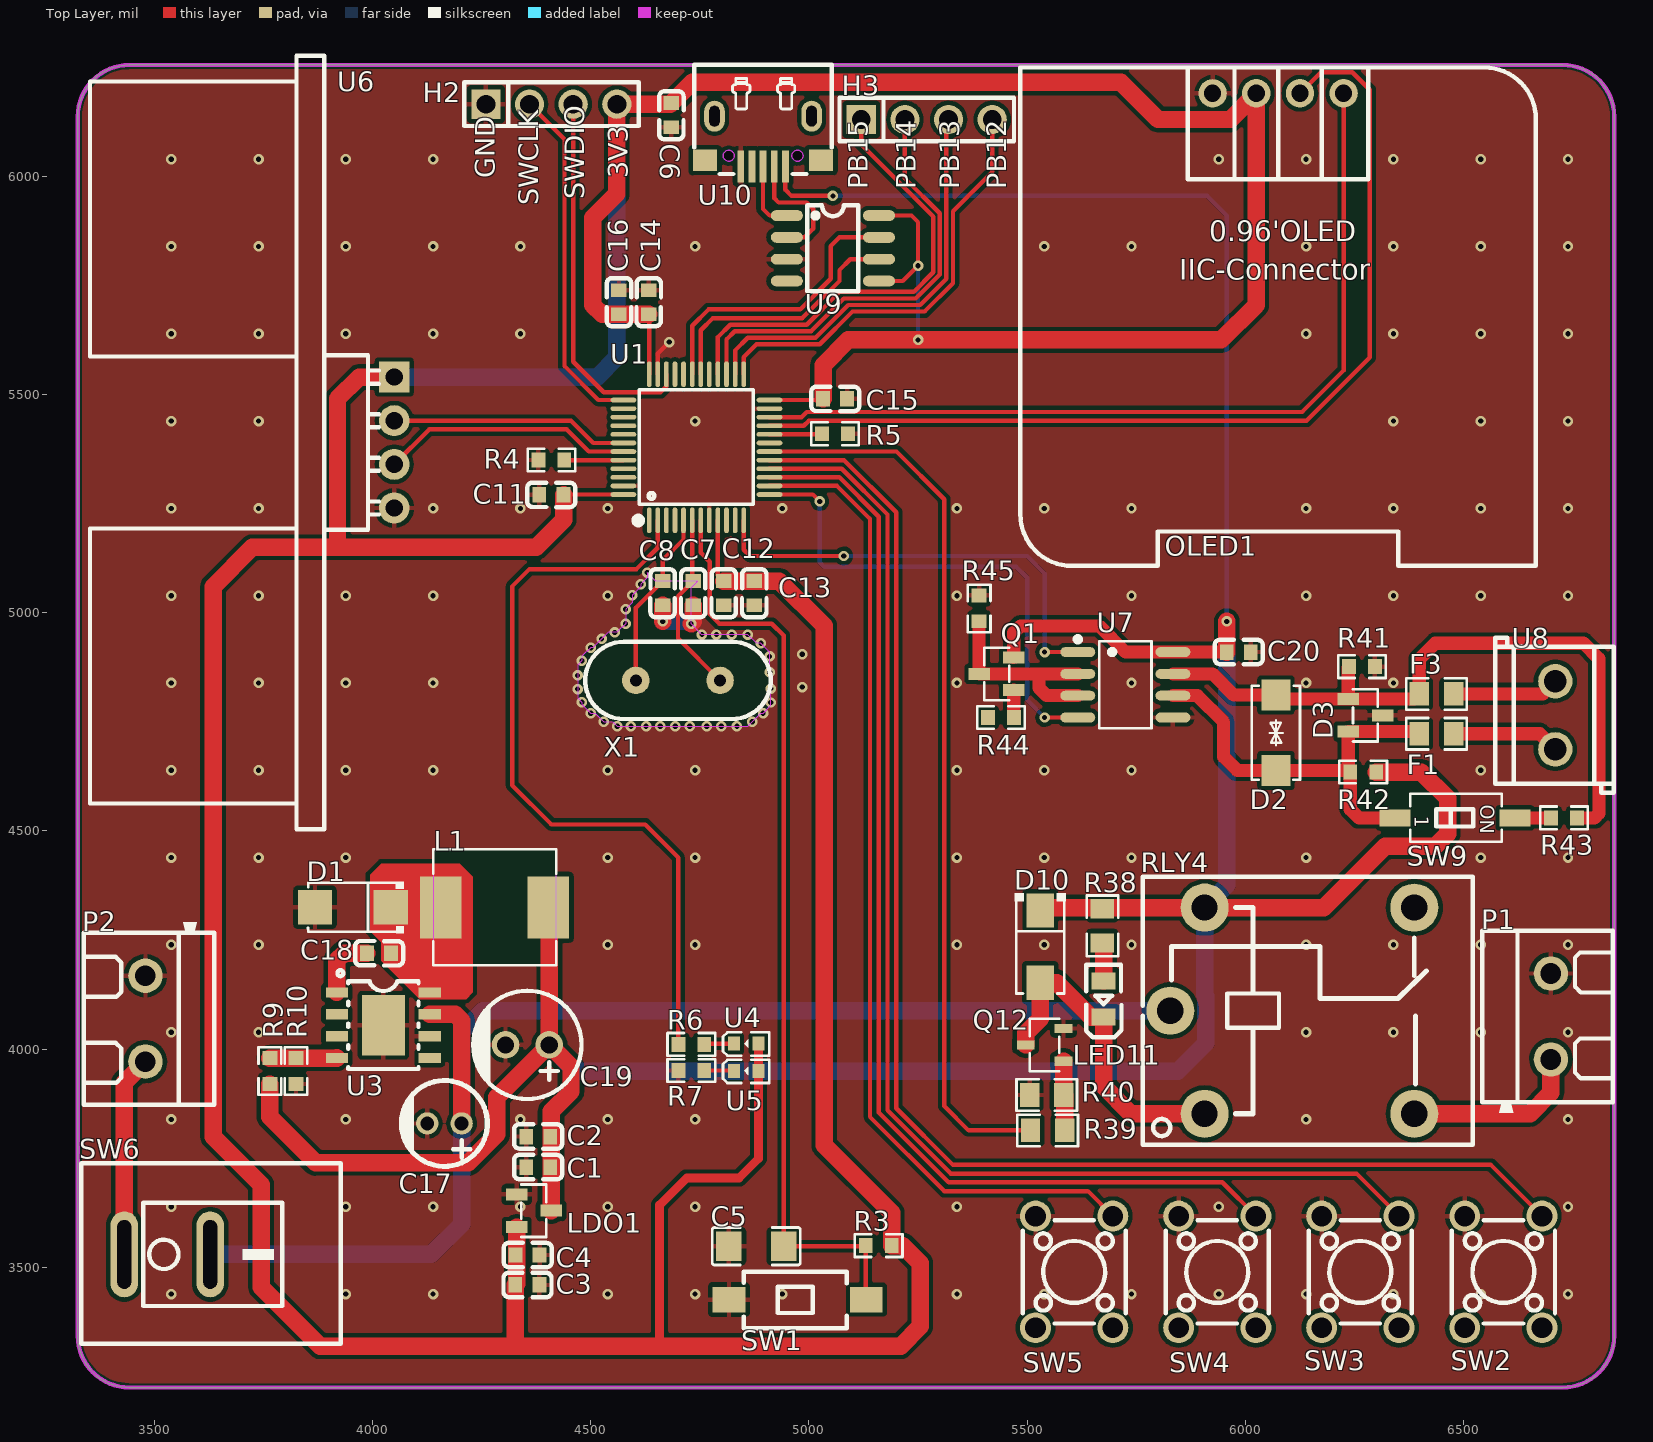
[diagram p0: Top Layer view]
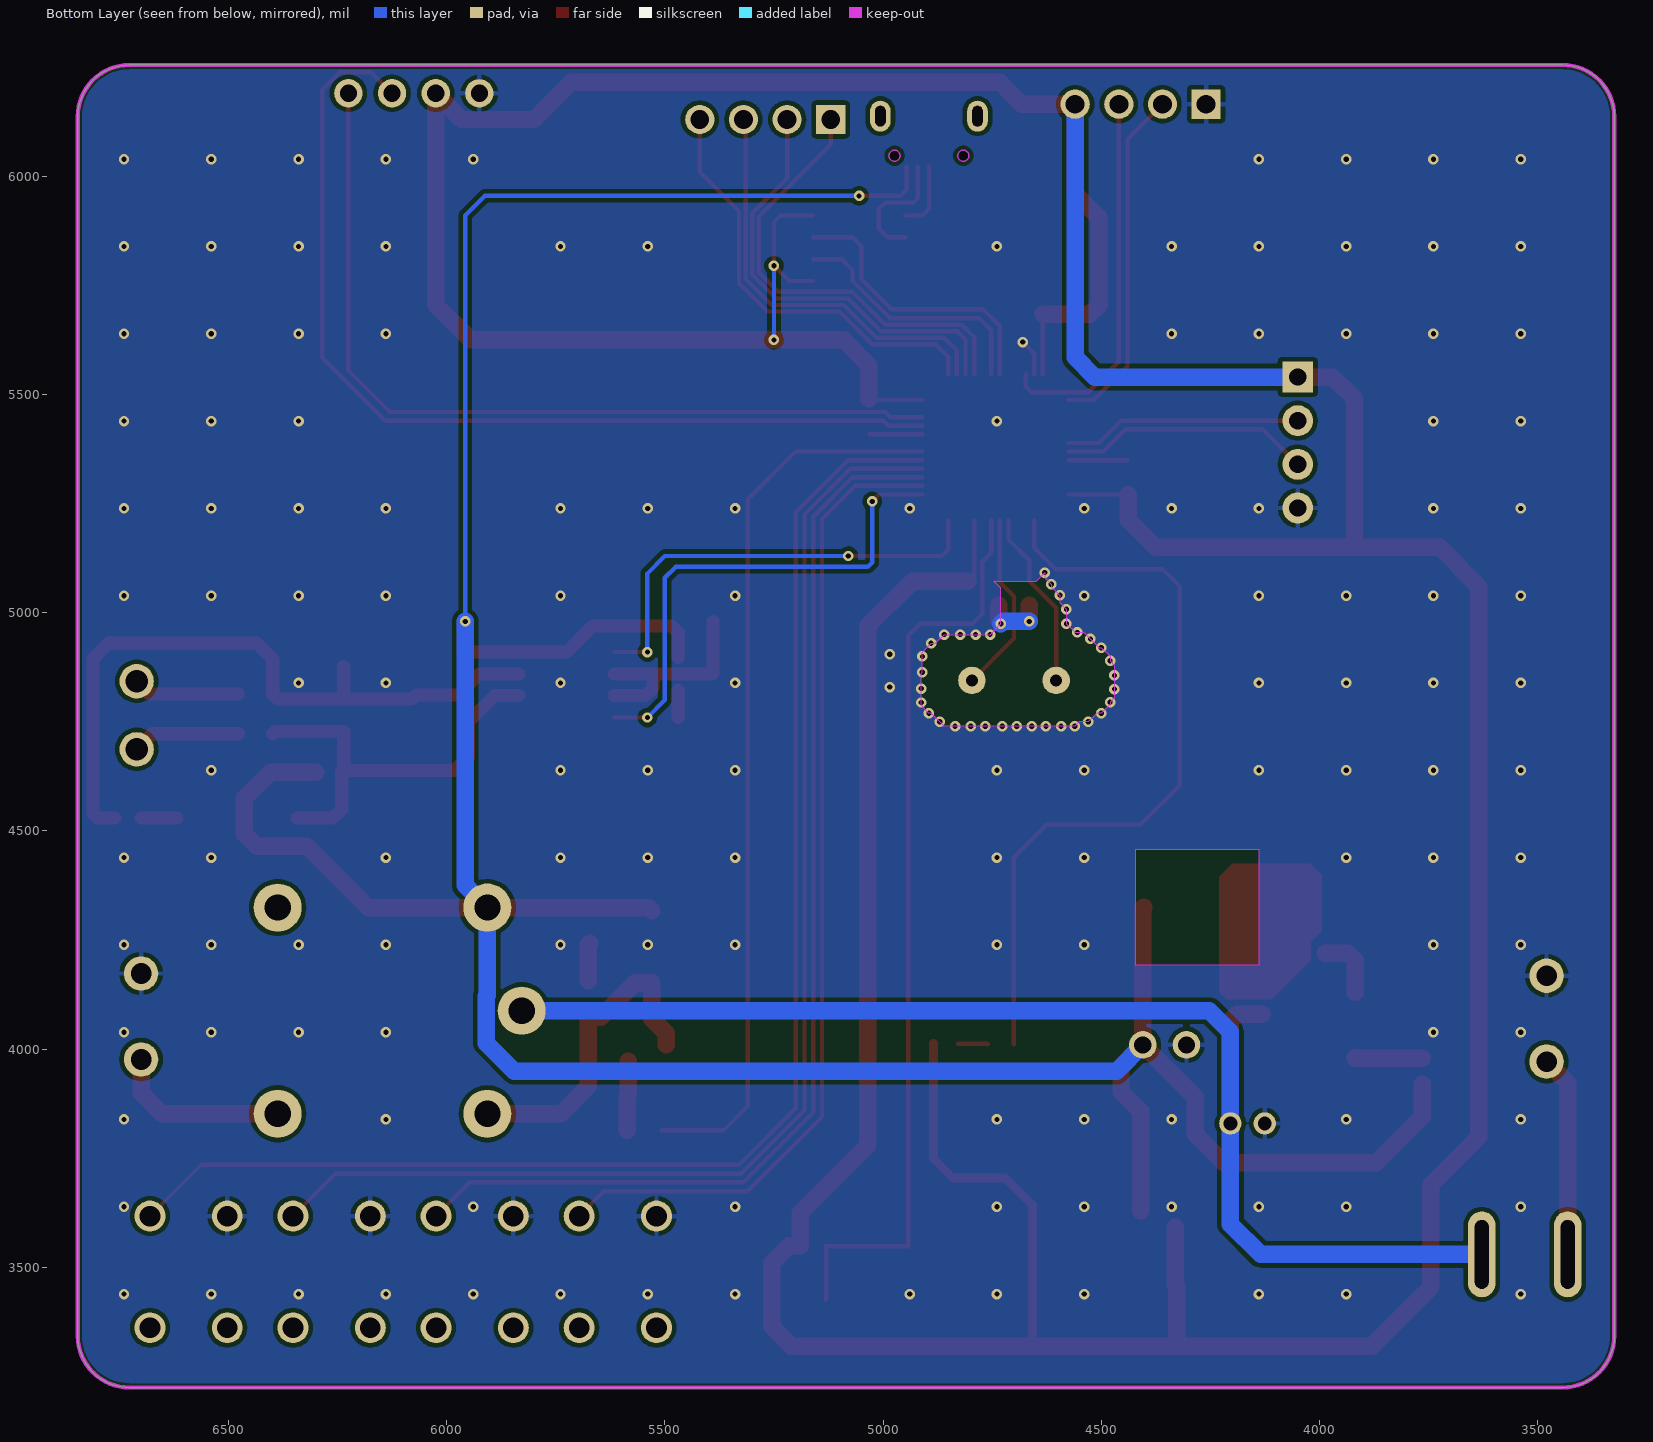
[diagram p1: Bottom Layer view, seen from below]
# Altium PCB MISC64779.pcbdoc
Units mil, origin at the board's own origin, x right, y up, seen from the top; angles counter-clockwise.
Board outline 3520 x 3030 mil, 2 copper layers (Top Layer, Bottom Layer), stack 62.206 mil thick; 67 components, 64 nets, 229 pads, 183 vias.

## Layer stack, top to bottom
Top Solder Mask Layer: solder mask 0.394, Dk 3.3
Top Layer: signal copper 1.379
Dielectric1: surface 59.449, FR4, Dk 4.5
Bottom Layer: signal copper 1.378
Bottom Solder Mask Layer: solder mask 0.394, Dk 3.3

## Board outline
3443.11,6255 ccw(c3443.11,6136.89) 3325,6136.89 3325,3343.11 ccw(c3443.11,3343.11) 3443.11,3225 6726.89,3225 ccw(c6726.89,3343.11) 6845,3343.11 6845,6136.89 ccw(c6726.89,6136.89) 6726.89,6255

## Design rules (kind name [scope] priority, off if disabled: settings)
BoardOutlineClearance copperThickness2oz_1 [All] p2 off: genericclearance=7.99 ignorepadtopadclearanceinfootprint=FALSE except(0: Arc-SplitContinuation Track-SplitContinuation SMDPad-SplitContinuation THPad-SplitContinuation Via-SplitContinuation Fill-SplitContinuation Region-SplitContinuation Poly-SplitContinuation Text-SplitContinuation Hole-SplitContinuation; 5.98: Arc-CutoutEdge Track-CutoutEdge SMDPad-CutoutEdge THPad-CutoutEdge Via-CutoutEdge Text-CutoutEdge; 6.9: Hole-OutlineEdge Hole-CutoutEdge; 10: Poly-OutlineEdge Poly-CutoutEdge; 11.81: Arc-OutlineEdge Track-OutlineEdge SMDPad-OutlineEdge THPad-OutlineEdge Via-OutlineEdge Fill-OutlineEdge Region-OutlineEdge Text-OutlineEdge Fill-CutoutEdge Region-CutoutEdge)
BoardOutlineClearance Plane_innerPlane_1 [All] p4 off: genericclearance=4.02 ignorepadtopadclearanceinfootprint=FALSE except(0: Arc-SplitContinuation Track-SplitContinuation SMDPad-SplitContinuation THPad-SplitContinuation Via-SplitContinuation Fill-SplitContinuation Region-SplitContinuation Poly-SplitContinuation Text-SplitContinuation Hole-SplitContinuation; 5.98: Arc-CutoutEdge Track-CutoutEdge SMDPad-CutoutEdge THPad-CutoutEdge Via-CutoutEdge Text-CutoutEdge; 6.9: Hole-OutlineEdge Hole-CutoutEdge; 10: Poly-OutlineEdge Poly-CutoutEdge; 11.81: Arc-OutlineEdge Track-OutlineEdge SMDPad-OutlineEdge THPad-OutlineEdge Via-OutlineEdge Fill-OutlineEdge Region-OutlineEdge Text-OutlineEdge Fill-CutoutEdge Region-CutoutEdge)
BoardOutlineClearance Copper_copperRegion_1 [All] p6 off: genericclearance=4.02 ignorepadtopadclearanceinfootprint=FALSE except(0: Arc-SplitContinuation Track-SplitContinuation SMDPad-SplitContinuation THPad-SplitContinuation Via-SplitContinuation Fill-SplitContinuation Region-SplitContinuation Poly-SplitContinuation Text-SplitContinuation Hole-SplitContinuation; 5.98: Arc-CutoutEdge Track-CutoutEdge SMDPad-CutoutEdge THPad-CutoutEdge Via-CutoutEdge Text-CutoutEdge; 6.9: Hole-OutlineEdge Hole-CutoutEdge; 10: Poly-OutlineEdge Poly-CutoutEdge; 11.81: Arc-OutlineEdge Track-OutlineEdge SMDPad-OutlineEdge THPad-OutlineEdge Via-OutlineEdge Fill-OutlineEdge Region-OutlineEdge Text-OutlineEdge Fill-CutoutEdge Region-CutoutEdge)
BoardOutlineClearance copperThickness1oz_1 [All] p8: genericclearance=4.02 ignorepadtopadclearanceinfootprint=FALSE except(0: Arc-SplitContinuation Track-SplitContinuation SMDPad-SplitContinuation THPad-SplitContinuation Via-SplitContinuation Fill-SplitContinuation Region-SplitContinuation Poly-SplitContinuation Text-SplitContinuation Hole-SplitContinuation; 5.98: Arc-CutoutEdge Track-CutoutEdge SMDPad-CutoutEdge THPad-CutoutEdge Via-CutoutEdge Text-CutoutEdge; 6.9: Hole-OutlineEdge Hole-CutoutEdge; 10: Poly-OutlineEdge Poly-CutoutEdge; 11.81: Arc-OutlineEdge Track-OutlineEdge SMDPad-OutlineEdge THPad-OutlineEdge Via-OutlineEdge Fill-OutlineEdge Region-OutlineEdge Text-OutlineEdge Fill-CutoutEdge Region-CutoutEdge)
Clearance copperThickness2oz [All] p1 off: gap=7.99 ignorepadtopadclearanceinfootprint=FALSE except(5.98: SMDPad-Track SMDPad-SMDPad THPad-Track SMDPad-THPad THPad-THPad Track-Via SMDPad-Via THPad-Via Via-Via Fill-SMDPad Region-SMDPad Fill-THPad Region-THPad Fill-Via Region-Via Fill-Fill Fill-Region Region-Region Arc-Track Arc-SMDPad Arc-THPad Arc-Via Fill-Arc Region-Arc Arc-Arc Text-Track SMDPad-Text Text-THPad Text-Via Fill-Text Region-Text Arc-Text Text-Text; 6.9: Hole-Track Hole-SMDPad Hole-THPad Hole-Via Fill-Hole Region-Hole Hole-Arc Hole-Text; 10: Poly-Track Poly-SMDPad Poly-THPad Poly-Via Poly-Fill Poly-Region Poly-Poly Poly-Arc Poly-Text Poly-Hole; 11.81: Fill-Track Region-Track)
Clearance Plane_innerPlane [All] p3 off: gap=4.02 ignorepadtopadclearanceinfootprint=FALSE except(5.98: SMDPad-Track SMDPad-SMDPad THPad-Track SMDPad-THPad THPad-THPad Track-Via SMDPad-Via THPad-Via Via-Via Fill-SMDPad Region-SMDPad Fill-THPad Region-THPad Fill-Via Region-Via Fill-Fill Fill-Region Region-Region Arc-Track Arc-SMDPad Arc-THPad Arc-Via Fill-Arc Region-Arc Arc-Arc Text-Track SMDPad-Text Text-THPad Text-Via Fill-Text Region-Text Arc-Text Text-Text; 6.9: Hole-Track Hole-SMDPad Hole-THPad Hole-Via Fill-Hole Region-Hole Hole-Arc Hole-Text; 10: Poly-Track Poly-SMDPad Poly-THPad Poly-Via Poly-Fill Poly-Region Poly-Poly Poly-Arc Poly-Text Poly-Hole; 11.81: Fill-Track Region-Track)
Clearance Copper_copperRegion [All] p5 off: gap=4.02 ignorepadtopadclearanceinfootprint=FALSE except(5.98: SMDPad-Track SMDPad-SMDPad THPad-Track SMDPad-THPad THPad-THPad Track-Via SMDPad-Via THPad-Via Via-Via Fill-SMDPad Region-SMDPad Fill-THPad Region-THPad Fill-Via Region-Via Fill-Fill Fill-Region Region-Region Arc-Track Arc-SMDPad Arc-THPad Arc-Via Fill-Arc Region-Arc Arc-Arc Text-Track SMDPad-Text Text-THPad Text-Via Fill-Text Region-Text Arc-Text Text-Text; 6.9: Hole-Track Hole-SMDPad Hole-THPad Hole-Via Fill-Hole Region-Hole Hole-Arc Hole-Text; 10: Poly-Track Poly-SMDPad Poly-THPad Poly-Via Poly-Fill Poly-Region Poly-Poly Poly-Arc Poly-Text Poly-Hole; 11.81: Fill-Track Region-Track)
Clearance copperThickness1oz [All] p7: gap=4.02 ignorepadtopadclearanceinfootprint=FALSE except(5.98: SMDPad-Track SMDPad-SMDPad THPad-Track SMDPad-THPad THPad-THPad Track-Via SMDPad-Via THPad-Via Via-Via Fill-SMDPad Region-SMDPad Fill-THPad Region-THPad Fill-Via Region-Via Fill-Fill Fill-Region Region-Region Arc-Track Arc-SMDPad Arc-THPad Arc-Via Fill-Arc Region-Arc Arc-Arc Text-Track SMDPad-Text Text-THPad Text-Via Fill-Text Region-Text Arc-Text Text-Text; 6.9: Hole-Track Hole-SMDPad Hole-THPad Hole-Via Fill-Hole Region-Hole Hole-Arc Hole-Text; 10: Poly-Track Poly-SMDPad Poly-THPad Poly-Via Poly-Fill Poly-Region Poly-Poly Poly-Arc Poly-Text Poly-Hole; 11.81: Fill-Track Region-Track)
DiffPairsRouting differentialPair [All] p1: maxlimit=6 minlimit=6 mostfreqgap=6 toplayer_minwidth=5 toplayer_prefwidth=10 toplayer_maxwidth=100 toplayer_mingap=6 toplayer_prefgap=6 toplayer_maxgap=6 bottomlayer_minwidth=5 bottomlayer_prefwidth=10 bottomlayer_maxwidth=100 bottomlayer_mingap=6 bottomlayer_prefgap=6 bottomlayer_maxgap=6 maxuncoupledlength=10
HoleToHoleClearance otherClearance [All] p1: gap=11.81 allowstackedmicrovias=TRUE
Length netLength [All] p1: minlimit=0 maxlimit=0
PasteMaskExpansion pasteMaskExpansion [All] p1: expansion=0
PlaneConnect innerPlane [All] p1: planeconnectstyle=Relief reliefexpansion=20 reliefentries=4 reliefconductorwidth=10 reliefairgap=10
PolygonConnect copperRegion [All] p1: connectstyle=Relief reliefconductorwidth=10 reliefentries=4 polygonreliefangle="90 Angle" airgapwidth=10 via.connectstyle=Relief via.reliefconductorwidth=10 via.reliefentries=4 via.polygonreliefangle="90 Angle" via.airgapwidth=10
RoutingVias viaSize [All] p1: holewidth=12.01 width=24.02 viastyle="Through Hole" minholewidth=11.81 minwidth=19.68 maxholewidth=248.03 maxwidth=393.7
SolderMaskExpansion solderMaskExpansion [IsVia] p1: expansion=-1000 istentingtop=TRUE
SolderMaskExpansion solderMaskExpansion [All] p2: expansion=2 istentingtop=FALSE
Width copperThickness2oz_2 [All] p1 off: maxlimit=100 minlimit=8 preferedwidth=10
Width copperThickness1oz_2 [All] p2: maxlimit=100 minlimit=5 preferedwidth=10

## Components (designator, comment, footprint, x,y, rotation, side; value= is the part's Value field where it differs from the comment)
C1 "10uF" C0603 4380,3730 r0 top
C2 "100nF" C0603 4380,3800 r0 top
C3 "100nF" C0603 4355,3460 r180 top
C4 "10uF" C0603 4355.51,3528.58 r180 top
C5 "100uF" C1206 4879.43,3548.58 r0 top
C6 "100nF" C0603 4685,6140 r90 top
C7 "20pF" C0603 4735,5045 r90 top
C8 "20pF" C0603 4665,5045 r90 top
C11 "100nF" C0603 4410,5270 r0 top
C12 "100nF" C0603 4805,5045 r90 top
C13 "100nF" C0603 4875,5045 r90 top
C14 "100nF" C0603 4632.98,5711.29 r270 top
C15 "100nF" C0603 5060,5490 r180 top
C16 "4.7nF" C0603 4564.8,5711.29 r270 top
C17 "10uF" CAP-TH_BD5.0-P2.00-D0.8-FD 4165,3830 r180 top
C18 "10nF" C0603 4015,4220 r180 top
C19 "220uF" CAP-TH_BD6.3-P2.50-D1.0-FD 4355,4010 r180 top
C20 "100nF" C0603 5985,4910 r0 top
D1 "B340A" SMA_L4.3-W2.6-LS5.1-RD 3955,4325 r180 top
D2 "SMAJ7.0CA" SMA_L4.5-W2.7-LS5.1-BI 6070,4725 r270 top
D3 "SM712" SOT-23-3_L2.9-W1.3-P1.90-LS2.4-BR 6275,4765 r180 top
D10 "1N4007" SMA_L4.3-W2.5-LS5.0-RD 5530,4235 r270 top
F1 "0R" R0805 6437.63,4722.67 r0 top
F3 "0R" R0805 6437.63,4814.14 r0 top
H2 "" HDR-TH_4P-P2.54-V-M 4410,6165 r0 top
H3 "" HDR-TH_4P-P2.54-V-M 5270,6130 r0 top
L1 "15uH" IND-SMD_L7.0-W6.6_FXL0630 4280,4325 r0 top
LDO1 "SC662K-3.3V" SOT-23-3_L2.9-W1.3-P1.90-LS2.4-BR 4370,3630 r180 top
LED11 "NCD0805R1" LED0805-R-RD 5675,4115 r90 top
OLED1 "" 0.96OLED_4P 6075,6190 r0 top
P1 "KF301-2P terminal block" CONN-TH_XY301V-A-5.0-2P 6700,4075 r270 top
P2 "KF301-2P terminal block" CONN-TH_XY301V-A-5.0-2P 3480,4070 r90 top
Q1 "S8550-2TY" SOT-23-3_L2.9-W1.3-P0.95-LS2.4-BR 5430,4860 r0 top
Q12 "S8050 J3Y(RANGE:200-350)" SOT-23-3_L3.0-W1.7-P0.95-LS2.9-BR 5540,4010 r0 top
R3 "1kΩ" R0603 5160,3550 r0 top
R4 "10kΩ" R0603 4410,5350 r0 top
R5 "10kΩ" R0603 5060,5410 r180 top
R6 "510Ω" R0603 4730.72,4011.18 r180 top
R7 "510Ω" R0603 4730.72,3951.18 r180 top
R9 "10kΩ" R0603 3765,3950 r90 top
R10 "3.24kΩ" R0603 3825,3950 r90 top
R38 "1.5kΩ" R0805 5672.28,4282.73 r90 top
R39 "1kΩ" R0805 5547.1,3814.1 r0 top
R40 "10kΩ" R0805 5545,3895 r0 top
R41 "3.3K" R0603 6266.95,4876.44 r180 top
R42 "3.3K" R0603 6270,4635 r0 top
R43 "120R" R0603 6730,4530 r0 top
R44 "4.7K" R0603 5440,4760 r0 top
R45 "10K" R0603 5390,5010 r90 top
RLY4 "SRD-05VDC-SL-C" RELAY-TH_SRD-XXVDC-XL-C 6107.46,4088.36 r0 top
SW1 "TS-1101-C-W" SW-SMD_L6.0-W3.3-LS8.0 4974.3,3426.3 r0 top
SW2 "" SW-TH_4P-L6.0-W6.0-P4.50-LS6.5 6591.06,3489.8 r270 top
SW3 "" SW-TH_4P-L6.0-W6.0-P4.50-LS6.5 6263.31,3489.8 r270 top
SW4 "" SW-TH_4P-L6.0-W6.0-P4.50-LS6.5 5935.55,3489.8 r270 top
SW5 "" SW-TH_4P-L6.0-W6.0-P4.50-LS6.5 5607.79,3489.8 r270 top
SW6 "KCD11-2P-R" SW-TH_2P-L15.0-W10.5-P5.00_KCD11-2P-R 3530,3530 r0 top
SW9 "ZX-1.27BM-1PSMD" SW-SMD_L5.4-W2.8-LS8.2 6480,4530 r270 top
U1 "STM32F103C8T6" LQFP-48_L7.0-W7.0-P0.50-LS9.0-BL 4742.36,5379.1 r0 top
U3 "TPS5430DDAR" ESOP-8_L4.9-W3.9-P1.27-LS6.0-TL-EP 4025,4055 r0 top
U4 "42-51/GHC-YW2X2K/3T" LED-SMD_L1.6-W0.8-FD_GREEN-1 4856.42,4012.9 r180 top
U5 "42-51/GHC-YW2X2K/3T" LED-SMD_L1.6-W0.8-FD_GREEN-1 4856.42,3950.25 r180 top
U6 "HC-SR04" TH_HC-SR04V 4050,5390 r270 top
U7 "MAX485ESA" SOP-8_L5.0-W4.0-P1.27-LS6.0-BL 5725,4835 r270 top
U8 "KF396-3.96-2P" CONN-TH_P3.96_KF396-3.96-2P 6710,4765 r90 top
U9 "CH340N" SOP-8_L4.9-W3.9-P1.27-LS6.0-BL 5055,5835 r270 top
U10 "micro-B USB socket" MICRO-USB_C9900039549 4895,6080 r180 top
X1 "8MHz" OSC-TH_L10.0-W4.5-P5.00 4700,4845 r90 top

## Footprints (in the part's own frame and the unit in brackets; to place one, negate y for a bottom-side part, rotate by r counter-clockwise, add the part's x,y. Pads: shape width x height; smd on the part's side, far side on the other; paste and mask are expansions set on the pad)
0.96OLED_4P [mm]
  round 1.65 hole 1 copper offset 0,0: 1(-3.81,-0.001) 2(-1.27,0.002) 3(1.27,0.002) 4(3.81,0.002)
  silkscreen extent -15,-27.5 15,1.5
C0603 [mm]
  rect 0.8x0.9 smd: 1(-0.7,0) 2(0.7,0)
  silkscreen extent -1.41,-0.71 1.39,0.72
C1206 [mm]
  rect 1.485x1.728 smd paste-100 mask+0.051: 1(-1.593,0) 2(1.593,0)
  silkscreen extent -2.56,-1.09 2.56,1.09
CAP-TH_BD5.0-P2.00-D0.8-FD [mm]
  round 1.3 hole 0.8: 1(-1,0) 2(1,0)
  silkscreen extent -2.5,-2.5 2.5,2.5
CAP-TH_BD6.3-P2.50-D1.0-FD [mm]
  round 1.6 hole 1: 1(-1.27,0) 2(1.27,0)
  silkscreen extent -3.15,-3.15 3.17,3.15
CONN-TH_P3.96_KF396-3.96-2P [mm]
  round 2 hole 1.3: 1(-1.98,0) 2(1.98,0)
  silkscreen extent -4.51,-3.4 4.51,3.5
CONN-TH_XY301V-A-5.0-2P [mm]
  round 2 hole 1.2: 1(-2.5,0) 2(2.5,0)
  silkscreen extent -5,-4 5.6,3.6
ESOP-8_L4.9-W3.9-P1.27-LS6.0-TL-EP [mm]
  rect 1.3x0.6 smd: 1(-2.7,1.905) 2(-2.7,0.635) 3(-2.7,-0.635) 4(-2.7,-1.905) 5(2.7,-1.905) 6(2.7,-0.635) 7(2.7,0.635) 8(2.7,1.905)
  rect 2.5x3.5 smd: 9(0,0)
  silkscreen extent -2.67,-2.55 2.05,3.2
HDR-TH_4P-P2.54-V-M [mm]
  rect 1.7x1.7 hole 1.1: 1(-3.81,0)
  round 1.7 hole 1.1: 2(-1.27,0) 3(1.27,0) 4(3.81,0)
  silkscreen extent -5.08,-1.27 5.08,1.27
IND-SMD_L7.0-W6.6_FXL0630 [mm]
  rect 2.424x3.62 smd: 1(3.128,0) 2(-3.128,0)
  silkscreen extent -3.58,-3.38 3.58,3.38
LED0805-R-RD [mm]
  rect 1x1.4 smd: 1(1.05,0) 2(-1.05,0)
  silkscreen extent -2.22,-1.04 1.99,1.01
LED-SMD_L1.6-W0.8-FD_GREEN-1 [mm]
  rect 0.7x0.8 smd: 1(-0.715,0) 2(0.715,0)
  silkscreen extent -1.35,-0.65 1.35,0.7
LQFP-48_L7.0-W7.0-P0.50-LS9.0-BL [mm]
  oval 0.27x1.5 smd paste+0 mask+0.05: 1(-2.75,-4.25) 2(-2.25,-4.25) 3(-1.75,-4.25) 4(-1.25,-4.25) 5(-0.75,-4.25) 6(-0.25,-4.25) 7(0.25,-4.25) 8(0.75,-4.25) 9(1.25,-4.25) 10(1.75,-4.25) 11(2.25,-4.25) 12(2.75,-4.25) 25(2.75,4.25) 26(2.25,4.25) 27(1.75,4.25) 28(1.25,4.25) 29(0.75,4.25) 30(0.25,4.25) 31(-0.25,4.25) 32(-0.75,4.25) 33(-1.25,4.25) 34(-1.75,4.25) 35(-2.25,4.25) 36(-2.75,4.25)
  oval 1.5x0.27 smd paste+0 mask+0.05: 13(4.25,-2.75) 14(4.25,-2.25) 15(4.25,-1.75) 16(4.25,-1.25) 17(4.25,-0.75) 18(4.25,-0.25) 19(4.25,0.25) 20(4.25,0.75) 21(4.25,1.25) 22(4.25,1.75) 23(4.25,2.25) 24(4.25,2.75) 37(-4.25,2.75) 38(-4.25,2.25) 39(-4.25,1.75) 40(-4.25,1.25) 41(-4.25,0.75) 42(-4.25,0.25) 43(-4.25,-0.25) 44(-4.25,-0.75) 45(-4.25,-1.25) 46(-4.25,-1.75) 47(-4.25,-2.25) 48(-4.25,-2.75)
  silkscreen extent -3.59,-4.46 3.3,3.34
MICRO-USB_C9900039549 [mm]
  rect 0.4x1.85 smd paste-100 mask+0.051: 1(-1.3,1.462) 2(-0.65,1.462) 3(0,1.462) 4(0.65,1.462) 5(1.3,1.462)
  rect 1.4x1.25 smd paste-100 mask+0.051: 6(-3.375,1.1) 7(3.375,1.1)
  oval 1.2x1.8 hole 0.6 slot 1.2 at 90 deg copper offset -0.001,0.001: 6(-2.824,-1.463)
  oval 1.2x1.8 hole 0.6 slot 1.2 at 90 deg copper offset -0.001,-0.001: 7(2.826,-1.462)
  Board Outline Layer circle w0.003: c2,0.837 r0.325
  Board Outline Layer circle w0.003: c-2,0.837 r0.325
  Board Outline Layer region: 1.675,0.837 1.707,0.978 1.797,1.091 1.928,1.154 2.072,1.154 2.203,1.091 2.293,0.978 2.325,0.837 2.325,0.837 2.293,0.696 2.203,0.583 2.072,0.52 1.928,0.52 1.797,0.583 1.707,0.696 1.675,0.837
  Board Outline Layer region: 1.675,0.837 1.684,0.915 1.712,0.988 1.757,1.053 1.815,1.105 1.885,1.141 1.961,1.16 2.039,1.16 2.115,1.141 2.185,1.105 2.243,1.053 2.288,0.988 2.316,0.915 2.325,0.837 2.316,0.76 2.288,0.686 2.243,0.622 2.185,0.57 2.115,0.533 2.039,0.515 1.961,0.515 1.885,0.533 1.815,0.57 1.757,0.622 1.712,0.686 1.684,0.76
  Board Outline Layer region: -2.325,0.837 -2.293,0.978 -2.203,1.091 -2.072,1.154 -1.928,1.154 -1.797,1.091 -1.707,0.978 -1.675,0.837 -1.675,0.837 -1.707,0.696 -1.797,0.583 -1.928,0.52 -2.072,0.52 -2.203,0.583 -2.293,0.696 -2.325,0.837
  Board Outline Layer region: -2.325,0.837 -2.316,0.915 -2.288,0.988 -2.243,1.053 -2.185,1.105 -2.115,1.141 -2.039,1.16 -1.961,1.16 -1.885,1.141 -1.815,1.105 -1.757,1.053 -1.712,0.988 -1.684,0.915 -1.675,0.837 -1.684,0.76 -1.712,0.686 -1.757,0.622 -1.815,0.57 -1.885,0.533 -1.961,0.515 -2.039,0.515 -2.115,0.533 -2.185,0.57 -2.243,0.622 -2.288,0.686 -2.316,0.76
  Multi-Layer board cut-out: 1.675,0.837 1.707,0.978 1.797,1.091 1.928,1.154 2.072,1.154 2.203,1.091 2.293,0.978 2.325,0.837 2.325,0.837 2.293,0.696 2.203,0.583 2.072,0.52 1.928,0.52 1.797,0.583 1.707,0.696 1.675,0.837
  Multi-Layer board cut-out: -2.325,0.837 -2.293,0.978 -2.203,1.091 -2.072,1.154 -1.928,1.154 -1.797,1.091 -1.707,0.978 -1.675,0.837 -1.675,0.837 -1.707,0.696 -1.797,0.583 -1.928,0.52 -2.072,0.52 -2.203,0.583 -2.293,0.696 -2.325,0.837
  silkscreen extent -4,-4.46 4,1.91
OSC-TH_L10.0-W4.5-P5.00 [mm]
  round 1.6 hole 0.7: 1(0,2.45) 2(0,-2.45)
  silkscreen extent -2.25,-5.39 2.25,5.39
R0603 [mil]
  rect 31.75x34.02 smd paste-3937.01 mask+2: 1(-29.66,0) 2(29.66,0)
  silkscreen extent -55,-26 55,26
R0805 [mm]
  rect 1.133x1.377 smd paste-100 mask+0.051: 1(-1,0) 2(1,0)
  silkscreen extent -1.76,-0.92 1.76,0.92
RELAY-TH_SRD-XXVDC-XL-C [mil]
  round 110 hole 60: 1(-200.79,-236.22) 2(279.53,-236.2) 3(279.53,236.2) 4(-200.79,236.22) 5(-279.53,0)
  silkscreen extent -342,-307 413,307
SMA_L4.3-W2.5-LS5.0-RD [mm]
  rect 2x1.593 smd: 1(-2.1,0) 2(2.1,0)
  silkscreen extent -3.11,-1.48 2.73,1.48
SMA_L4.3-W2.6-LS5.1-RD [mm]
  rect 2x2 smd: 1(-2.2,0) 2(2.2,0)
  silkscreen extent -2.98,-1.5 2.6,1.5
SMA_L4.5-W2.7-LS5.1-BI [mm]
  rect 1.8x1.7 smd: 1(-2.192,0) 2(2.192,0)
  silkscreen extent -2.73,-1.4 2.73,1.4
SOP-8_L4.9-W3.9-P1.27-LS6.0-BL [mm]
  oval 0.63x1.865 smd: 1(-1.905,-2.682) 2(-0.635,-2.682) 3(0.635,-2.682) 4(1.905,-2.682) 5(1.905,2.682) 6(0.635,2.682) 7(-0.635,2.682) 8(-1.905,2.682)
  silkscreen extent -2.5,-1.5 2.5,1.48
SOP-8_L5.0-W4.0-P1.27-LS6.0-BL [mil]
  oval 22.6x80.14 smd: 1(-75,-108.97) 2(-25,-108.97) 3(25,-108.97) 4(75,-108.97) 5(75,108.97) 6(25,108.97) 7(-25,108.97) 8(-75,108.97)
  silkscreen extent -110,-115 99,60
SOT-23-3_L2.9-W1.3-P0.95-LS2.4-BR [mm]
  rect 1.25x0.7 smd: 1(1,-0.95) 2(1,0.95) 3(-1,0)
  silkscreen extent -0.73,-1.53 0.73,1.53
SOT-23-3_L2.9-W1.3-P1.90-LS2.4-BR [mm]
  rect 1.25x0.7 smd: 1(1,-0.95) 2(1,0.95) 3(-1,0)
  silkscreen extent -0.73,-1.53 0.73,1.53
SOT-23-3_L3.0-W1.7-P0.95-LS2.9-BR [mil]
  rect 40.85x20.95 smd: 1(43.36,-37.4) 2(43.36,37.4) 3(-43.36,0)
  silkscreen extent -34,-60 34,60
SW-SMD_L5.4-W2.8-LS8.2 [mm]
  rect 1x1.8 smd paste+0 mask+0.05: 1(0,-3.492) 2(0,3.492)
  silkscreen extent -1.4,-2.6 1.4,2.73
SW-SMD_L6.0-W3.3-LS8.0 [mm]
  rect 1.9x1.5 smd: 1(-4,0) 2(4,0)
  silkscreen extent -3.14,-1.67 2.86,1.63
SW-TH_2P-L15.0-W10.5-P5.00_KCD11-2P-R [mm]
  oval 1.6x5 hole 0.8 slot 4 at 90 deg: 1(-2.5,0) 2(2.5,0)
  silkscreen extent -5,-5.2 10.1,5.3
SW-TH_4P-L6.0-W6.0-P4.50-LS6.5 [mm]
  round 1.8 hole 1.2: 1(-3.25,2.25) 2(3.25,2.25) 3(-3.25,-2.25) 4(3.25,-2.25)
  silkscreen extent -3,-3 3,3
TH_HC-SR04V [mm]
  rect 1.8x1.8 hole 1.001: 1(-3.81,0)
  round 1.8 hole 1.001: 2(-1.27,0) 3(1.27,0) 4(3.81,0)
  silkscreen extent -22.5,-17.7 22.5,-0.89

## Via types
v1: diameter 24.02, hole 12, Top Layer to Bottom Layer, 176 vias
v2: diameter 24, hole 12, Top Layer to Bottom Layer, 7 vias

## Nets (pads, with @x,y where several pads share a name; then routed paths per layer and width w, separated by ;. In a path a pad name is that pad's centre, name@x,y a point inside that pad or via, vN(x,y) a via of type N, cw(c..) or ccw(c..) an arc to the next point about the centre after c; other vN are vias at no path point)
3V3: C3.2 C4.2 C6.2 C11.2 C12.2 C13.2 C14.2 C15.2 C16.2 H2.4 LDO1.2 OLED1.2 R3.2 U1.9 U1.24 U1.36 U1.48 U4.1 U5.1 U6.1 U9.5 U9.8 | length 13664.4
  Top Layer w10: C11.2 4438.39,5270.83 U1.48 ; C14.2 4634.09,5682.62 U1.36 ; U1.9 4791.57,5085.99 C12.2 ; U1.24 5029.81,5487.37 C15.2 ; U9.5 5215,5760 v1(5250,5795) 5250,5895 5235,5910 U9.8
  Top Layer w20: 4657.95,3320 4657.95,3642.95 4720,3705 4840,3705 4884.57,3749.57 U5.1 U4.1
  Top Layer w40: U6.1 3970,5540 3920,5490 3920,5150 ; LDO1.2 4330.63,3463.19 C3.2 4327.44,3320 ; C11.2@4438.39,5270.83 4438.39,5213.39 4375,5150 3920,5150 ; C14.2 C16.2 4526.27,5683.73 4505,5705 4505,5905 4560,5960 H2.4 4682.44,6165 C6.2 4732.44,6215 5715,6215 5800,6130 5964.95,6130 6025,6190.05 6025,5705 5945,5625 v1(5250,5625) 5090,5625 5032.44,5567.44 C15.2 ; C12.2 C13.2 4932.44,5072.56 5035,4970 5035,3780 5189.66,3625.34 R3.2 5215,3550 5255,3510 5255,3365 5210,3320 4657.95,3320 4327.44,3320 ; 3920,5150 3725,5150 3635,5060 3635,3800 3745,3690 3745,3455 3880,3320 4327.44,3320
  Bottom Layer w10: v1(5250,5625) v1(5250,5795)
  Bottom Layer w40: U6.1 4515,5540 4560,5585 H2.4
$1N2099: R6.1 U4.2 | length 68.6
  Top Layer w10: R6.1 4762.1,4012.9 U4.2
$1N2100: R7.1 U5.2 | length 68.3
  Top Layer w10: R7.1 4827.34,3951.18 U5.2
$1N3320: C18.2 U3.1 | length 149.2
  Top Layer w40: U3.1 3918.7,4203.7 3935,4220 C18.2
$1N3323: R9.2 R10.2 U3.4 | length 153.8
  Top Layer w40: R9.2 R10.2 3918.36,3979.66 U3.4
$1N3325: C18.1 D1.1 L1.2 U3.8
$1N3655: D10.2 LED11.2 Q12.3 RLY4.1 | length 750.1
  Top Layer w40: Q12.3 5496.64,4036.64 5530,4070 D10.2 5567.68,4152.32 5646.35,4073.65 LED11.2 5675,3915 5737.86,3852.14 RLY4.1
$1N3657: LED11.1 R38.1 | length 88.1
  Top Layer w40: R38.1 5675,4240.65 LED11.1
$1N3658: Q12.1 R39.2 R40.2 | length 159.8
  Top Layer w40: Q12.1 5584.37,3971.59 R40.2 5586.47,3892.9 R39.2
$1N4325: R43.1 SW9.2 | length 82.8
  Top Layer w30: SW9.2 R43.1
$1N4326: F1.2 U8.1 | length 247.8
  Top Layer w30: F1.2 6674.38,4722.67 U8.1
$1N4327: F3.2 U8.2 | length 244.9
  Top Layer w30: F3.2 6681.19,4814.14 U8.2
$1N4341: Q1.3 R45.1 U7.2 U7.3 | length 474.5
  Top Layer w30: R45.1 5390,4860.63 Q1.3 5527.02,4860 ; U7.3 5545,4810 5527.02,4827.98 5527.02,4860 ; U7.2 5527.02,4860
$1N4344: Q1.1 R44.2 | length 62.7
  Top Layer w30: Q1.1 5469.37,4760.29 R44.2
$1N4387: P2.1 SW6.1 | length 461.6
  Top Layer w40: SW6.1 3431.57,3923.15 P2.1
$1N8218: U9.1 U10.3 | length 158
  Top Layer w10: U10.3 4895,5925 4910,5910 U9.1
$1N8222: U9.2 U10.2 | length 286.1
  Top Layer w10: U10.2 4920.6,5950 4930.6,5940 4995,5940 5010,5925 5010,5880 4990,5860 U9.2
+5V: C1.2 C2.2 C19.1 C20.1 D10.1 L1.1 LDO1.3 Q1.2 R9.1 R38.2 R42.2 RLY4.4 U7.8 U10.1 | length 8140.9
  Top Layer w10: U10.1 4946.2,5968.8 4960,5955 v1(5055,5955)
  Top Layer w30: Q1.2 5469.37,4954.37 5485,4970 5665,4970 5725,4910 U7.8 C20.1
  Top Layer w40: R9.1 3765,3845 3870,3740 4220,3740 4285,3805 4285,3890 C19.1 ; L1.1 4405,4323.15 C19.1 ; LDO1.3 4409.37,3857.52 4455,3903.15 4455,3960 C19.1 ; D10.1 5536.9,4324.58 RLY4.4 6179.58,4324.58 6320,4465 6435,4465 6463.28,4493.28 6463.28,4575 6403.28,4635 R42.2 ; C20.1 v2(5957.44,4980)
  Bottom Layer w10: v1(5055,5955) 5912.44,5955 5957.44,5910 v2(5957.44,4980)
  Bottom Layer w40: C19.1 4465,3950 5845,3950 5908.91,4013.91 5908.91,4121.91 5906.67,4124.15 RLY4.4 5957.44,4375.35 v2(5957.44,4980)
A: D2.2 D3.2 F1.1 R42.1 SW9.1 U7.6 | length 970.2
  Top Layer w30: U7.6 5890,4810 5950,4750 5950,4670 5981.31,4638.69 D2.2 6236.65,4638.69 6235.63,4639.71 D3.2 6393.33,4727.6 F1.1 ; R42.1 6240.34,4549.66 6260,4530 SW9.1
B: D2.1 D3.1 F3.1 R41.2 R43.2 U7.7 | length 1597.8
  Top Layer w30: U7.7 5925,4860 5973.69,4811.31 D2.1 6078.91,4802.4 D3.1 ; R41.2 6235.63,4874.78 D3.1 ; R43.2 6800,4530 6810,4540 6810,4895 6775,4930 6435,4930 6398.26,4893.26 F3.1 6386.51,4802.4 D3.1
BOOT0: R4.2 U1.44 | length 135.6
  Top Layer w10: R4.2 4440.09,5349.57 U1.44
BOOT1: R5.2 U1.20 | length 121.2
  Top Layer w10: U1.20 5028.97,5408.63 R5.2
CLK: H2.2 U1.37 | length 800.3
  Top Layer w10: H2.2 4440,6085 4440,5565 4517.63,5487.37 U1.37
DIO: H2.3 U1.34 | length 866
  Top Layer w10: H2.3 4460,5575 4530,5505 4660,5505 4673.46,5518.46 U1.34
GND: C1.1 C2.1 C3.1 C4.1 C5.1 C6.1 C7.1 C8.1 C11.1 C12.1 C13.1 C14.1 C15.1 C16.1 C17.2 C19.2 C20.2 D1.2 D3.3 H2.1 LDO1.1 OLED1.1 P1.1 P2.2 Q12.2 R4.1 R5.1 R7.2 R10.1 R40.1 R41.1 R45.2 SW1.1 SW2.3 SW3.3 SW4.3 SW5.3 U1.8 U1.23 U1.35 U1.47 U3.6 U3.9 U6.4 U7.5 U9.3 U10.5 | length 233.5
  Top Layer w10: U1.35 4653.78,5593.78 v2(4680,5620)
  Top Layer w40: v2(4665,4980) C8.1 ; v1(4730,4975) 4735,4980 C7.1
  Bottom Layer w40: v2(4665,4980) 4725,4980 v1(4730,4975)
  other v1: 3539.1,3439.1 3939.1,3439.1 4139.1,3439.1 4539.1,3439.1 4739.1,3439.1 4939.1,3439.1 5339.1,3439.1 5539.1,3439.1 5739.1,3439.1 5939.1,3439.1 6139.1,3439.1 6339.1,3439.1 6539.1,3439.1 6739.1,3439.1 3539.1,3639.1 3939.1,3639.1 4139.1,3639.1 4339.1,3639.1 4539.1,3639.1 4739.1,3639.1 5339.1,3639.1 5939.1,3639.1 6739.1,3639.1 3539.1,3839.1 3939.1,3839.1 4339.1,3839.1 4539.1,3839.1 4739.1,3839.1 6139.1,3839.1 6739.1,3839.1 3539.1,4039.1 3739.1,4039.1 6139.1,4039.1 6339.1,4039.1 6539.1,4039.1 6739.1,4039.1 3539.1,4239.1 3739.1,4239.1 4539.1,4239.1 4739.1,4239.1 5339.1,4239.1 5539.1,4239.1 5739.1,4239.1 6139.1,4239.1 6339.1,4239.1 6539.1,4239.1 6739.1,4239.1 3539.1,4439.1 3739.1,4439.1 3939.1,4439.1 4539.1,4439.1 4739.1,4439.1 5339.1,4439.1 5539.1,4439.1 5739.1,4439.1 6139.1,4439.1 6539.1,4439.1 6739.1,4439.1 3539.1,4639.1 3739.1,4639.1 3939.1,4639.1 4139.1,4639.1 4539.1,4639.1 4739.1,4639.1 5339.1,4639.1 5539.1,4639.1 5739.1,4639.1 6539.1,4639.1 4561.16,4740 4592.19,4740 4626.96,4740 4659.42,4740 4693.76,4740 4726.94,4740 4765.87,4740 4799.35,4740 4835,4740 4530,4750 4870,4750 4500,4770 4895,4770 4912.5,4794.36 4480,4795 4470,4825 4912.5,4826.21 4985,4829.84 3539.1,4839.1 3739.1,4839.1 3939.1,4839.1 4139.1,4839.1 5339.1,4839.1 5739.1,4839.1 6139.1,4839.1 6339.1,4839.1 4470,4856.28 4910.52,4863.6 4480,4890 4910,4900 4985,4905 4500,4920 4890,4930 4525,4940 4755,4950 4788.11,4950 4823.02,4950 4860.11,4950 4555,4955 4580,4975 4580,5008.13 3539.1,5039.1 3739.1,5039.1 3939.1,5039.1 4139.1,5039.1 4539.1,5039.1 5339.1,5039.1 5739.1,5039.1 6139.1,5039.1 6339.1,5039.1 6539.1,5039.1 6739.1,5039.1 4595,5040 4615,5065 4629.62,5092.11 3539.1,5239.1 3739.1,5239.1 4139.1,5239.1 4339.1,5239.1 4539.1,5239.1 4939.1,5239.1 5339.1,5239.1 5539.1,5239.1 5739.1,5239.1 6139.1,5239.1 6339.1,5239.1 6539.1,5239.1 6739.1,5239.1 3539.1,5439.1 3739.1,5439.1 4739.1,5439.1 6339.1,5439.1 6539.1,5439.1 6739.1,5439.1 3539.1,5639.1 3739.1,5639.1 3939.1,5639.1 4139.1,5639.1 4339.1,5639.1 6139.1,5639.1 6339.1,5639.1 6539.1,5639.1 6739.1,5639.1 3539.1,5839.1 3739.1,5839.1 3939.1,5839.1 4139.1,5839.1 4339.1,5839.1 4739.1,5839.1 5539.1,5839.1 5739.1,5839.1 6139.1,5839.1 6339.1,5839.1 6539.1,5839.1 6739.1,5839.1 3539.1,6039.1 3739.1,6039.1 3939.1,6039.1 4139.1,6039.1 5939.1,6039.1 6139.1,6039.1 6339.1,6039.1 6539.1,6039.1 6739.1,6039.1
OSC32-IN: U1.3
OSC32-OUT: U1.4
OSC-IN: C8.2 U1.5 X1.1 | length 412
  Top Layer w10: X1.1 4603.54,5011.1 C8.2 4665,5120 4712.83,5167.83 U1.5
OSC-OUT: C7.2 U1.6 X1.2 | length 422.3
  Top Layer w10: U1.6 4732.52,5075.04 C7.2 4700,5037.56 4700,4941.46 X1.2
PA0: U1.10
PA1: U1.11
PA2: U1.12 U7.1 | length 1035.3
  Top Layer w10: U1.12 4850.63,5144.37 4865,5130 v2(5080,5130) ; v2(5540,4910) U7.1
  Bottom Layer w10: v2(5080,5130) 5500,5130 5540,5090 v2(5540,4910)
PA3: U1.13 U7.4 | length 1164
  Top Layer w10: U1.13 5009.17,5270.83 v2(5025,5255) ; v2(5540,4760) U7.4
  Bottom Layer w10: v2(5025,5255) 5025,5115 5035,5105 5475,5105 5500,5080 5500,4800 v2(5540,4760)
PA4: SW5.1 U1.14 | length 2282.1
  Top Layer w10: U1.14 5064.48,5290.52 5140,5215 5140,3845 5310,3675 5639.12,3675 SW5.1
PA5: SW4.1 U1.15 | length 2615.1
  Top Layer w10: U1.15 5069.8,5310.2 5160,5220 5160,3855 5320,3695 5946.88,3695 SW4.1
PA6: SW3.1 U1.16 | length 2951
  Top Layer w10: U1.16 5075.11,5329.89 5180,5225 5180,3860 5325,3715 6254.64,3715 SW3.1
PA7: SW2.1 U1.17 | length 3286.9
  Top Layer w10: U1.17 5080.43,5349.57 5200,5230 5200,3865 5330,3735 6562.4,3735 SW2.1
PA8: U1.29
PA9: U1.30 U9.6 | length 591.3
  Top Layer w10: U1.30 4752.2,5647.2 4780,5675 4985,5675 5070,5760 5070,5785 5095,5810 U9.6
PA10: U1.31 U9.7 | length 667
  Top Layer w10: U1.31 4732.52,5657.52 4770,5695 4980,5695 5050,5765 5050,5840 5070,5860 U9.7
PA11: U1.32
PA12: U1.33
PA15: U1.38
PB0: R39.1 U1.18 | length 2056.5
  Top Layer w10: U1.18 5200.74,5369.26 5310,5260 5310,3870 5365.9,3814.1 R39.1
PB1: U1.19
PB3: U1.39
PB4: U1.40
PB5: U1.41
PB6: U1.42 U6.2 | length 546.2
  Top Layer w10: U6.2 4455,5440 4506.06,5388.94 U1.42
PB7: U1.43 U6.3 | length 579.2
  Top Layer w10: U6.3 4130,5420 4445,5420 4495.74,5369.26 U1.43
PB8: U1.45
PB9: U1.46
PB10: OLED1.3 U1.21 | length 2249.9
  Top Layer w10: U1.21 4988.31,5428.31 5000,5440 6140,5440 6285,5585 6285,6198.19 6245,6238.19 6173.14,6238.19 OLED1.3@6125,6190.05
PB11: OLED1.4 U1.22 | length 1994.7
  Top Layer w10: U1.22 4983,5448 4995,5460 6130,5460 6225,5555 OLED1.4@6225,6190.05
PB12: H3.4 U1.25 | length 1001
  Top Layer w10: U1.25 4850.63,5585.63 4880,5615 5025,5615 5100,5690 5265,5690 5330,5755 5330,5920 5420,6010 H3.4
PB13: H3.3 U1.26 | length 973.6
  Top Layer w10: U1.26 4830.94,5600.94 4860,5630 5015,5630 5090,5705 5255,5705 5315,5765 5315,6125 H3.3
PB14: H3.2 U1.27 | length 1018.3
  Top Layer w10: U1.27 4811.26,5626.26 4830,5645 5005,5645 5080,5720 5245,5720 5300,5775 5300,5915 5220,5995 H3.2
PB15: H3.1 U1.28 | length 1058.4
  Top Layer w10: U1.28 4791.57,5631.57 4820,5660 4995,5660 5070,5735 5240,5735 5285,5780 5285,5907.57 5120,6072.57 H3.1
PC13: R6.2 U1.2 | length 1766.2
  Top Layer w10: U1.2 4653.78,5148.78 4605,5100 4360,5100 4320,5060 4320,4605 4410,4515 4625,4515 4701.06,4438.94 R6.2
REST: C5.2 R3.1 SW1.2 U1.7 | length 2125.2
  Top Layer w10: U1.7 4752.2,5137.8 4772.93,5117.07 4772.93,4997.07 4795,4975 4915,4975 4942.13,4947.87 C5.2 5128.92,3548.58 R3.1 5130.34,3427.74 SW1.2
RLY4_OUT: P1.2 RLY4.2 | length 409.4
  Top Layer w40: RLY4.2 6652.16,3852.16 6700,3900 P1.2
TXD: R44.1
VBAT: U1.1
VCC: C17.1 RLY4.5 SW6.2 U3.7 | length 3004.1
  Top Layer w40: U3.7 4190,4080 4205,4065 4205,3830.63 C17.1
  Bottom Layer w40: SW6.2 4135,3530 4204.37,3599.37 C17.1 4204.37,4040 4252.73,4088.36 RLY4.5
pads on no net: RLY4.3 SW2.2 SW2.4 SW3.2 SW3.4 SW4.2 SW4.4 SW5.2 SW5.4 U3.2 U3.3 U3.5 U9.4 U10.4 U10.6 U10.7

## Polygon pours and split planes (outlines as drawn)
GND on Top Layer (solid, remove dead copper, pour order 0): 3000,6620 3000,3000 7110,3000 7110,6620
GND on Bottom Layer (solid, remove dead copper, pour order 2): 3100,6560 3100,3015 7075,3015 7075,6560

## Keep-outs
Board Outline Layer:
  region: 4629.62,5092.11 4629.62,5079.62 4615,5065 4615,5060 4595,5040 4595,5023.13 4580,5008.13 4580,4975 4560,4955 4540,4955 4505,4920 4500,4920 4480,4900 4480,4890 4470,4880 4470,4805 4480,4795 4480,4790 4500,4770 4510,4770 4530,4750 4551.16,4750 4561.16,4740 4860,4740 4890,4770 4895,4770 4912.5,4787.5 4912.5,4861.62 4910.52,4863.6 4910.52,4899.48 4910,4900 4910,4910 4890,4930 4880.11,4930 4860.11,4950 4755,4950 4730,4975 4730,5057.3 4745.26,5072.56 4649.17,5072.56
  region: 4139.2,4457.92 4139.2,4192.08 4420.8,4192.08 4420.8,4457.92
  lines w10: 3325,3343.11 3325,6136.89 cw(c3443.11,6136.89) 3443.11,6255 6726.89,6255 cw(c6726.89,6136.89) 6845,6136.89 6845,3343.11 cw(c6726.89,3343.11) 6726.89,3225 3443.11,3225 cw(c3443.11,3343.11) 3325,3343.11

## Other copper
Top Layer:
  region net $1N3325: 3995,4400 3995,4270 4020.3,4244.69 4020.3,4202.74 4108.04,4115 4215,4115 4230,4130 4230,4395 4200,4425 4020,4425

## Silkscreen, mask and mechanical layers (free items; w line width, h text height)
Top Silkscreen Layer:
  text "GND" at 4280,5995 h45 r90
  text "3V3" at 4585,5995 h45 r90
  text "PB12" at 5452.5,5970.6 h45 r90
  text "PB15" at 5135,5970 h45 r90
  text "PB14" at 5245,5970 h45 r90
  text "PB13" at 5345,5970 h45 r90
  text "SWDIO" at 4485,5946.9 h45 r90
  text "SWCLK" at 4380,5933.6 h45 r90